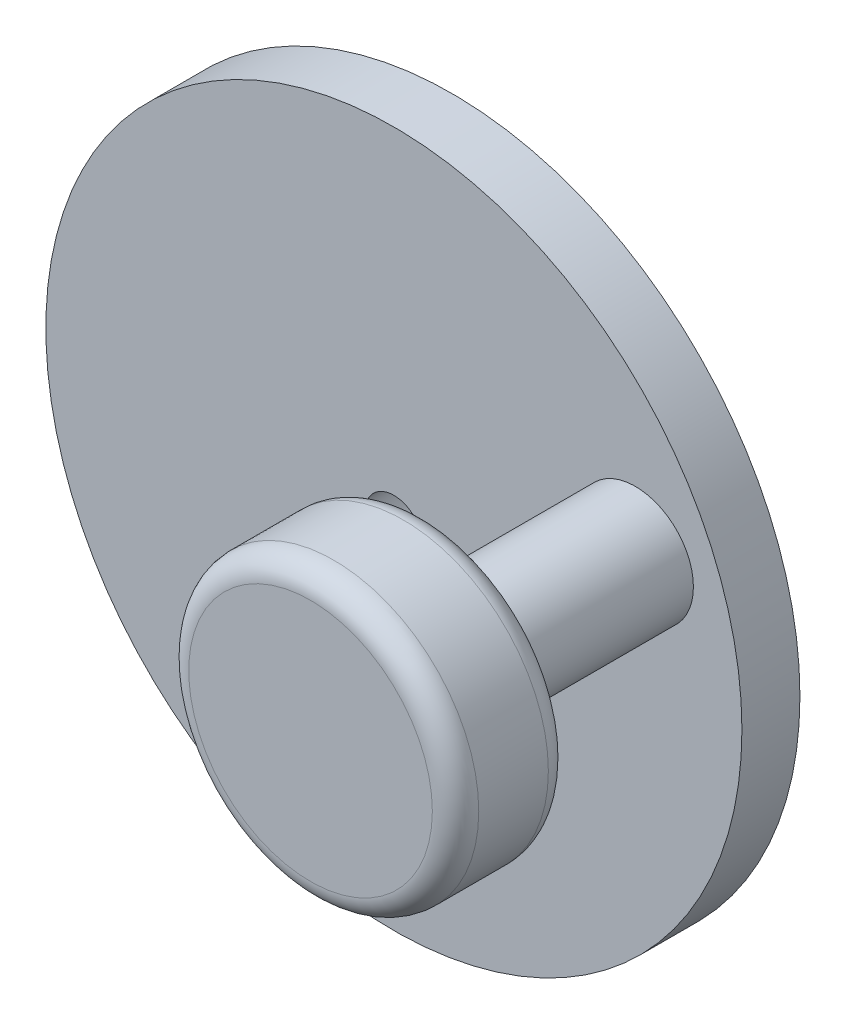
from build123d import *

# Parameters (mm, degrees)
SKETCH1_R           = 30
BOSS_EXTRUDE1_DEPTH = 5
SKETCH2_R           = 2.5
CUT_EXTRUDE1_DEPTH  = 5
SKETCH3_R           = 5
BOSS_EXTRUDE2_DEPTH = 18
SKETCH4_R           = 12.5
BOSS_EXTRUDE3_DEPTH = 10
FILLET1_R           = 2


with BuildPart() as part:
    # Sketch1 → Boss-Extrude1 (new body)
    with BuildSketch(Plane.XY):
        Circle(SKETCH1_R)
    extrude(amount=BOSS_EXTRUDE1_DEPTH)

    # Sketch2 → Cut-Extrude1 (cut)
    with BuildSketch(Plane.XY.offset(5)):
        Circle(SKETCH2_R)
    extrude(amount=-CUT_EXTRUDE1_DEPTH, mode=Mode.SUBTRACT)

    # Sketch3 → Boss-Extrude2 (add)
    with BuildSketch(Plane.XY.offset(5)):
        with Locations((20.816087355, 8.573414189)):
            Circle(SKETCH3_R)
    extrude(amount=BOSS_EXTRUDE2_DEPTH)

    # Sketch4 → Boss-Extrude3 (add)
    with BuildSketch(Plane.XY.offset(23)):
        with Locations((20.816087355, 8.573414189)):
            Circle(SKETCH4_R)
    extrude(amount=BOSS_EXTRUDE3_DEPTH)

    # Fillet1
    fillet1_edges = [part.edges().sort_by_distance(p)[0] for p in [
        (8.316087355, 8.573414189, 23),
        (8.316087355, 8.573414189, 33),
    ]]
    fillet(fillet1_edges, radius=FILLET1_R)


solid = part.part
